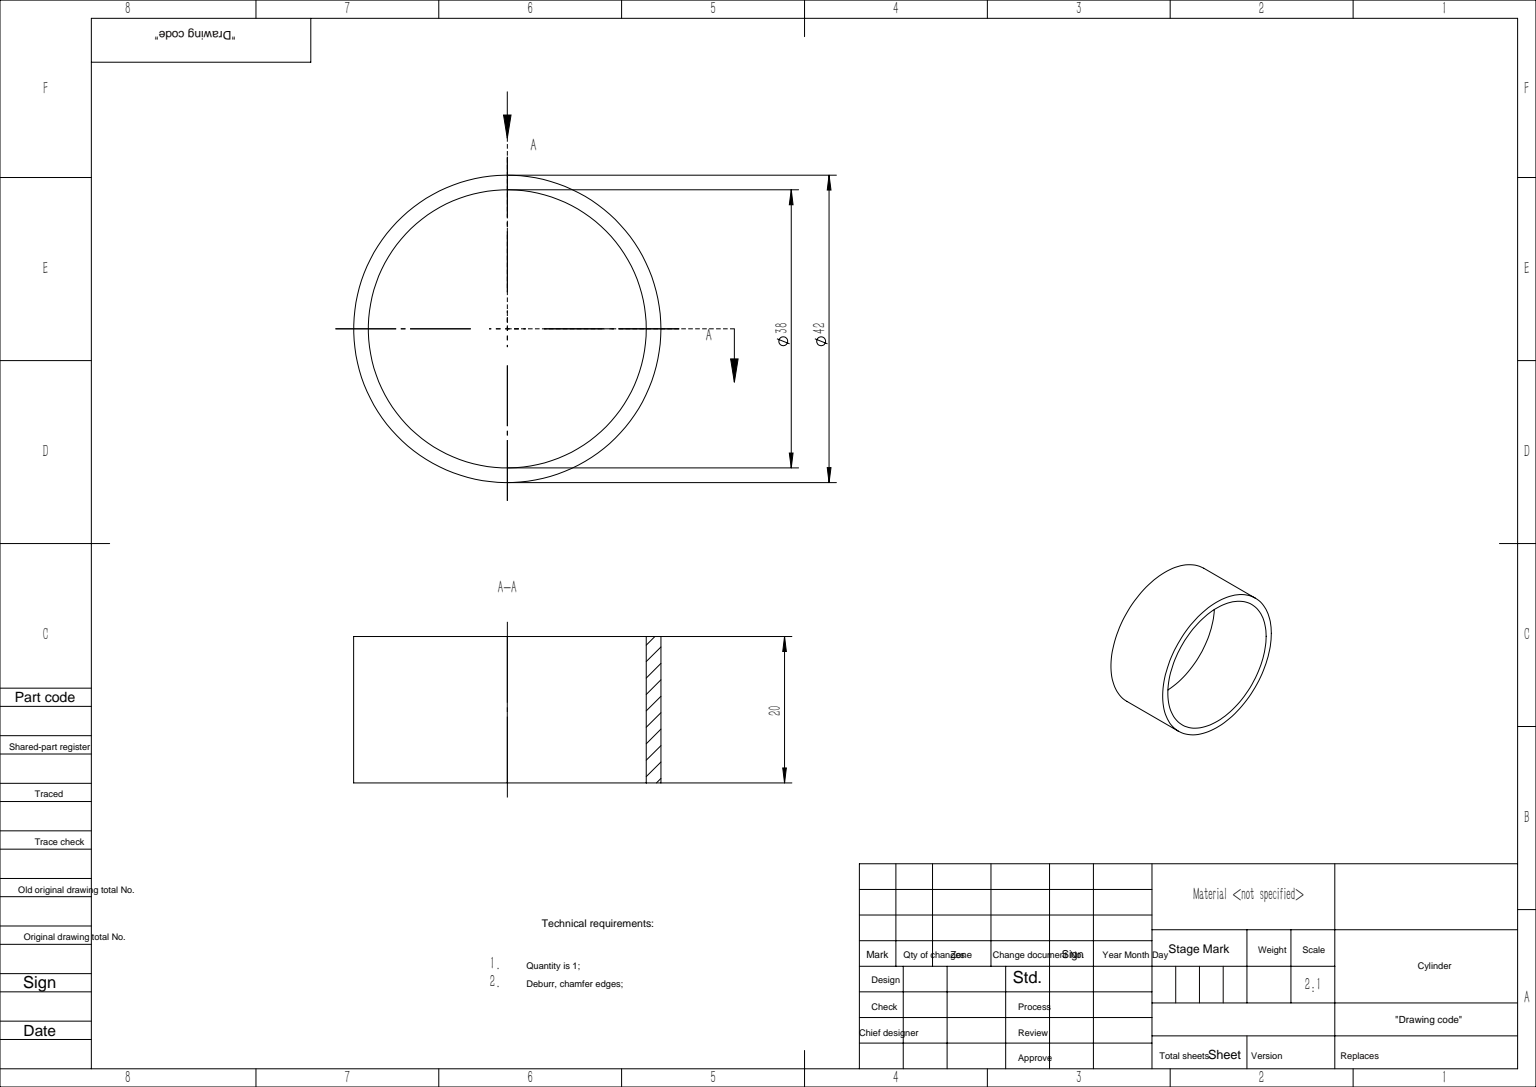
SolidWorks part; units mm, degrees
ref_plane "前视基准面" through (0, 0, 0) normal (0, 0, 1) x (1, 0, 0)
ref_plane "上视基准面" through (0, 0, 0) normal (0, 1, 0) x (1, 0, 0)
ref_plane "右视基准面" through (0, 0, 0) normal (1, 0, 0) x (0, 0, -1)
sketch "草图1" plane through (629.7, 0, 0) normal (1, 0, 0) x (0, 0, -1)
  circle A0 centre (201, -379) radius 19
  circle A1 centre (201, -379) radius 21
  dimension "D1" = 38
  dimension "D2" = 42
extrude "凸台-拉伸1" add sketch "草图1" along normal blind 20
